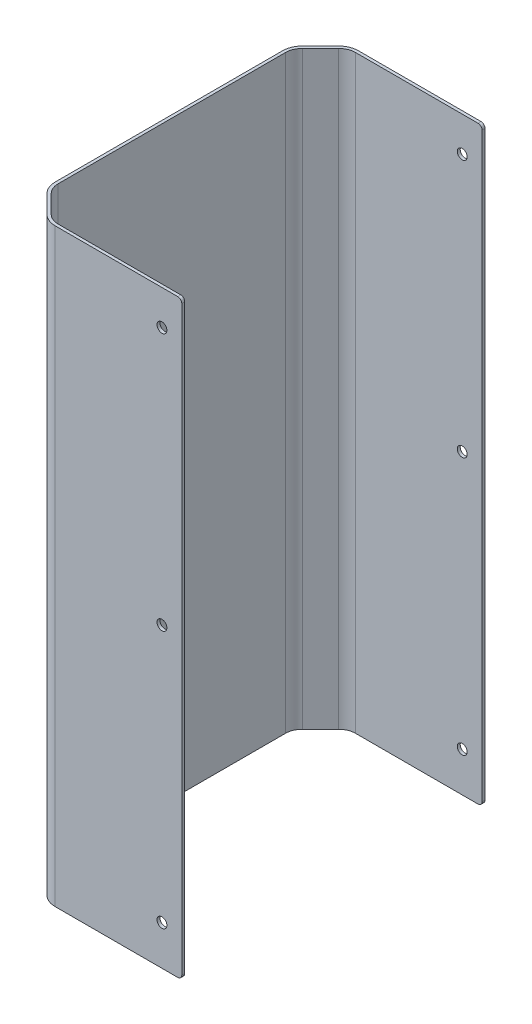
from build123d import *

# Parameters (mm, degrees)
SKETCH_2_W            = 83
SKETCH_2_H            = 153
EXTRUDE_2_DEPTH       = 297.5
CHAMFER_1_SIZE        = 15
FILLET_1_R            = 10
SHELL_2_T             = -1.5
HOLE_WIZARD_5_0_5_1_D = 5
FILLET_2_R            = 2


with BuildPart() as part:
    # 草图2 → 凸台-拉伸2 (new body)
    with BuildSketch(Plane(origin=(0, 0, 0), x_dir=(1, 0, 0), z_dir=(0, 1, 0))):
        Rectangle(SKETCH_2_W, SKETCH_2_H)
    extrude(amount=-EXTRUDE_2_DEPTH)

    # 倒角1
    chamfer_1_edges = [part.edges().sort_by_distance(p)[0] for p in [
        (-41.5, -148.75, 76.5),
        (-41.5, -148.75, -76.5),
    ]]
    chamfer(chamfer_1_edges, length=CHAMFER_1_SIZE)

    # 圆角1
    fillet_1_edges = [part.edges().sort_by_distance(p)[0] for p in [
        (-26.5, -148.75, -76.5),
        (-41.5, -148.75, 61.5),
        (-41.5, -148.75, -61.5),
        (-26.5, -148.75, 76.5),
    ]]
    fillet(fillet_1_edges, radius=FILLET_1_R)

    # 抽壳2
    shell_2_openings = [part.faces().sort_by_distance(p)[0] for p in [
        (0.682002961, -297.5, 0),
        (0.682002961, 0, 0),
        (41.5, -148.75, 0),
    ]]
    offset(amount=SHELL_2_T, openings=shell_2_openings, kind=Kind.INTERSECTION)

    # Ø5.0 (5) 直径孔1 (through all)
    with Locations(Plane.XY.offset(76.5)):
        with Locations((31.5, -17.5), (31.5, -147.5), (31.5, -277.5)):
            Hole(HOLE_WIZARD_5_0_5_1_D / 2)

    # 圆角2
    fillet_2_edges = [part.edges().sort_by_distance(p)[0] for p in [
        (41.5, -297.5, 75.75),
        (41.5, 0, -75.75),
        (41.5, -297.5, -75.75),
        (41.5, 0, 75.75),
    ]]
    fillet(fillet_2_edges, radius=FILLET_2_R)


solid = part.part
